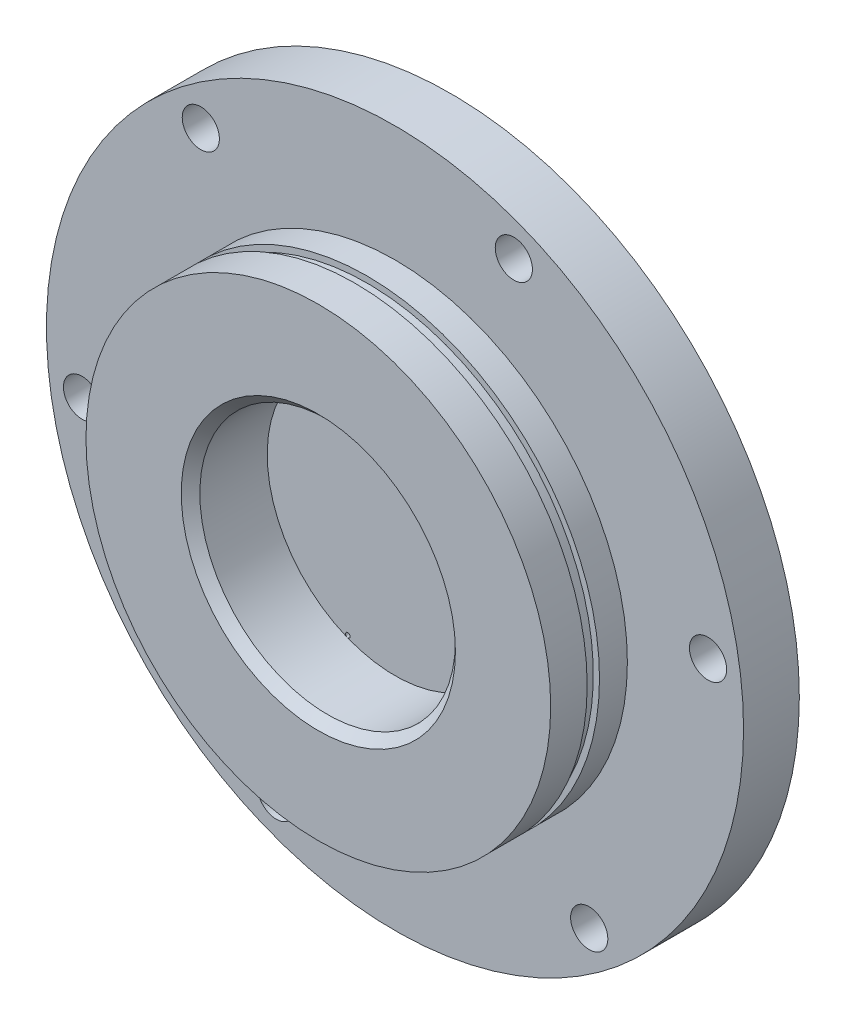
from build123d import *

# Parameters (mm, degrees)
SKETCH1_R           = 75
BOSS_EXTRUDE1_DEPTH = 12
SKETCH2_R           = 50
SKETCH2_R_2         = 27.5
BOSS_EXTRUDE2_DEPTH = 28.5
CUT_EXTRUDE1_START  = -18
SKETCH3_R           = 50
SKETCH3_R_2         = 48.675
CUT_EXTRUDE1_DEPTH  = 2.65
CHAMFER1_SIZE       = 2
SKETCH7_R           = 4
CUT_EXTRUDE2_DEPTH  = 110.828275048
SKETCH10_R          = 2.5
CUT_EXTRUDE3_DEPTH  = 7
SKETCH12_R          = 0.5
CUT_EXTRUDE8_DEPTH  = 109.223149095


with BuildPart() as part:
    # Sketch1 → Boss-Extrude1 (new body)
    with BuildSketch(Plane.XY):
        Circle(SKETCH1_R)
    extrude(amount=BOSS_EXTRUDE1_DEPTH)

    # Sketch2 → Boss-Extrude2 (add)
    with BuildSketch(Plane.XY):
        with Locations(Location((0, 0, 0), (0, 0, 180))):
            Circle(SKETCH2_R)
        with Locations(Location((0, 0, 0), (0, 0, 180))):
            Circle(SKETCH2_R_2, mode=Mode.SUBTRACT)
    extrude(amount=BOSS_EXTRUDE2_DEPTH)

    # Sketch3 → Cut-Extrude1 (cut)
    with BuildSketch(Plane(origin=(0, 0, 0), x_dir=(-1, 0, 0), z_dir=(0, 0, -1)).offset(CUT_EXTRUDE1_START)):
        Circle(SKETCH3_R)
        Circle(SKETCH3_R_2, mode=Mode.SUBTRACT)
    extrude(amount=-CUT_EXTRUDE1_DEPTH, mode=Mode.SUBTRACT)

    # Chamfer1
    chamfer1_edges = [part.edges().sort_by_distance(p)[0] for p in [
        (27.5, 0, 28.5),
    ]]
    chamfer(chamfer1_edges, length=CHAMFER1_SIZE)

    # Sketch7 → Cut-Extrude2 (cut, through all)
    with BuildSketch(Plane(origin=(0, 0, 0), x_dir=(-1, 0, 0), z_dir=(0, 0, -1))):
        with Locations((-25.564662216, 63.011491379)):
            Circle(SKETCH7_R)
        with Locations((41.787221156, 53.645392608)):
            Circle(SKETCH7_R)
        with Locations((67.351883372, -9.366098771)):
            Circle(SKETCH7_R)
        with Locations((25.564662216, -63.011491379)):
            Circle(SKETCH7_R)
        with Locations((-41.787221156, -53.645392608)):
            Circle(SKETCH7_R)
        with Locations((-67.351883372, 9.366098771)):
            Circle(SKETCH7_R)
    extrude(amount=-CUT_EXTRUDE2_DEPTH, mode=Mode.SUBTRACT)

    # Sketch10 → Cut-Extrude3 (cut)
    with BuildSketch(Plane(origin=(0, 0, 0), x_dir=(-1, 0, 0), z_dir=(0, 0, -1))):
        with Locations((10.150674704, -25.019268636)):
            Circle(SKETCH10_R)
    extrude(amount=-CUT_EXTRUDE3_DEPTH, mode=Mode.SUBTRACT)

    # Sketch12 → Cut-Extrude8 (cut, through all)
    with BuildSketch(Plane(origin=(0, 0, 7), x_dir=(-1, 0, 0), z_dir=(0, 0, -1))):
        with Locations((10.150674704, -25.019268636)):
            Circle(SKETCH12_R)
    extrude(amount=-CUT_EXTRUDE8_DEPTH, mode=Mode.SUBTRACT)


solid = part.part
